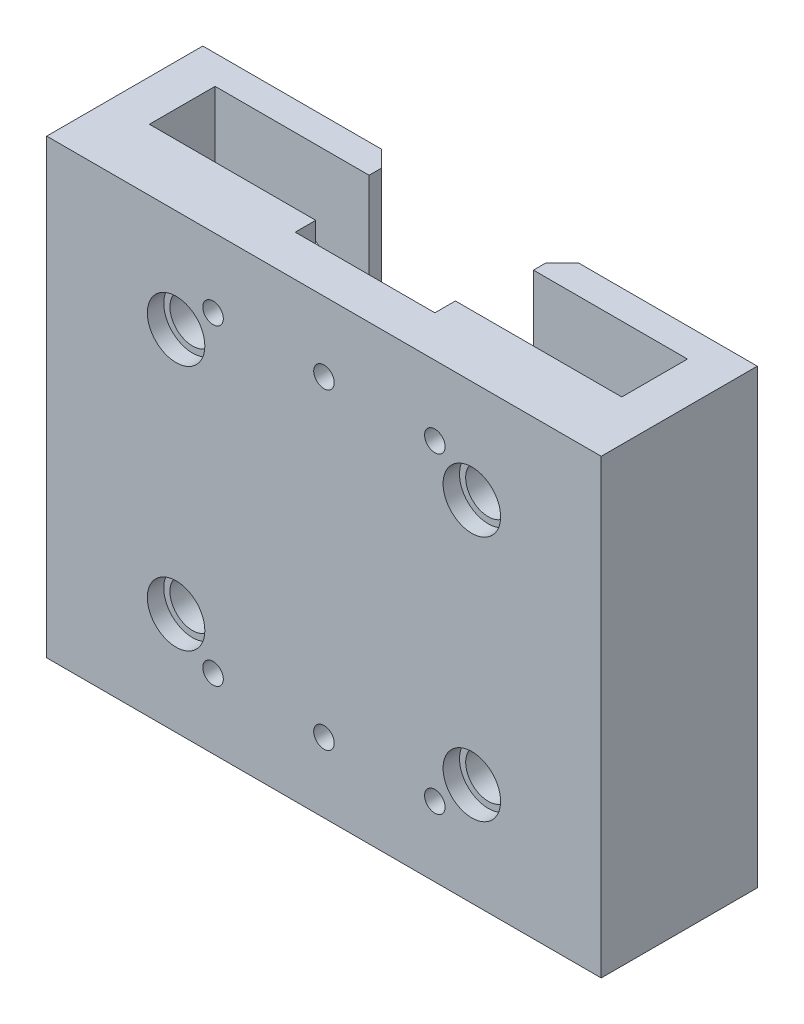
from build123d import *

# Parameters (mm, degrees)
SKETCH_1_W                  = 135
SKETCH_1_H                  = 38
EXTRUDE_1_DEPTH             = 110
CUT_EXTRUDE_1_DEPTH         = 131.450182062
SKETCH_4_R                  = 11
CUT_EXTRUDE_2_DEPTH         = 4
SKETCH_5_R                  = 5.5
CUT_EXTRUDE_3_DEPTH         = 134.462541561
SKETCH_6_R                  = 7
CUT_EXTRUDE_4_DEPTH         = 4
PATTERN_LINEAR_1_COUNT      = 2
PATTERN_LINEAR_1_PITCH      = 60
PATTERN_LINEAR_1_COUNT_DIR2 = 2
PATTERN_LINEAR_1_PITCH_DIR2 = 72
PATTERN_LINEAR_2_COUNT      = 3
PATTERN_LINEAR_2_PITCH      = 27
PATTERN_LINEAR_2_COUNT_DIR2 = 2
PATTERN_LINEAR_2_PITCH_DIR2 = 76
CHAMFER_1_SIZE              = 4


with BuildPart() as part:
    # 草图1 → 凸台-拉伸1 (new body)
    with BuildSketch(Plane(origin=(0, 0, 0), x_dir=(1, 0, 0), z_dir=(0, 1, 0))):
        Rectangle(SKETCH_1_W, SKETCH_1_H)
    extrude(amount=EXTRUDE_1_DEPTH)

    # 草图3 → 切除-拉伸1 (cut, through all)
    with BuildSketch(Plane(origin=(0, 110, 0), x_dir=(1, 0, 0), z_dir=(0, 1, 0))):
        Polygon((20, 19), (-20, 19), (-20, 12), (-57.5, 12), (-57.5, -4), (-17, -4), (-17, -9), (17, -9), (17, -4), (57.5, -4), (57.5, 12), (20, 12), align=None)
    extrude(amount=-CUT_EXTRUDE_1_DEPTH, mode=Mode.SUBTRACT)

    # 草图4 → 切除-拉伸2 (cut)
    with BuildSketch(Plane(origin=(0, 0, -19), x_dir=(-1, 0, 0), z_dir=(0, 0, -1))):
        with Locations((-36, 85)):
            Circle(SKETCH_4_R)
    cut_extrude_2 = extrude(amount=-CUT_EXTRUDE_2_DEPTH, mode=Mode.SUBTRACT)

    # 草图5 → 切除-拉伸3 (cut, through all)
    with BuildSketch(Plane(origin=(0, 0, -15), x_dir=(-1, 0, 0), z_dir=(0, 0, -1))):
        with Locations((-36, 85)):
            Circle(SKETCH_5_R)
    cut_extrude_3 = extrude(amount=-CUT_EXTRUDE_3_DEPTH, mode=Mode.SUBTRACT)

    # 草图6 → 切除-拉伸4 (cut)
    with BuildSketch(Plane.XY.offset(19)):
        with Locations((36, 85)):
            Circle(SKETCH_6_R)
    cut_extrude_4 = extrude(amount=-CUT_EXTRUDE_4_DEPTH, mode=Mode.SUBTRACT)

    # 阵列(线性)1: 切除-拉伸2, 切除-拉伸3, Cut-Extrude 4 2 × 2
    with Locations(*[(-j * PATTERN_LINEAR_1_PITCH_DIR2, -i * PATTERN_LINEAR_1_PITCH, 0) for i in range(PATTERN_LINEAR_1_COUNT) for j in range(PATTERN_LINEAR_1_COUNT_DIR2) if (i, j) != (0, 0)]):
        add(cut_extrude_2, mode=Mode.SUBTRACT)
        add(cut_extrude_3, mode=Mode.SUBTRACT)
        add(cut_extrude_4, mode=Mode.SUBTRACT)

    # 草图7 → M6 螺纹孔1 (revolve, cut)
    with BuildSketch(Plane(origin=(27, 93, 19), x_dir=(0, -1, 0), z_dir=(1, 0, 0))):
        Polygon((0, 0), (0, 13.443375673), (2.5, 12), (2.5, 0), align=None)
    hole_wizard_m6_1 = revolve(axis=Axis((27, 93, 25.35), (0, 0, -1)), mode=Mode.SUBTRACT)

    # 阵列(线性)2: Hole Wizard M6 _1 3 × 2
    with Locations(*[(-i * PATTERN_LINEAR_2_PITCH, -j * PATTERN_LINEAR_2_PITCH_DIR2, 0) for i in range(PATTERN_LINEAR_2_COUNT) for j in range(PATTERN_LINEAR_2_COUNT_DIR2) if (i, j) != (0, 0)]):
        add(hole_wizard_m6_1, mode=Mode.SUBTRACT)

    # 倒角1
    chamfer_1_edges = [part.edges().sort_by_distance(p)[0] for p in [
        (-20, 55, -19),
        (20, 55, -19),
    ]]
    chamfer(chamfer_1_edges, length=CHAMFER_1_SIZE)


solid = part.part
